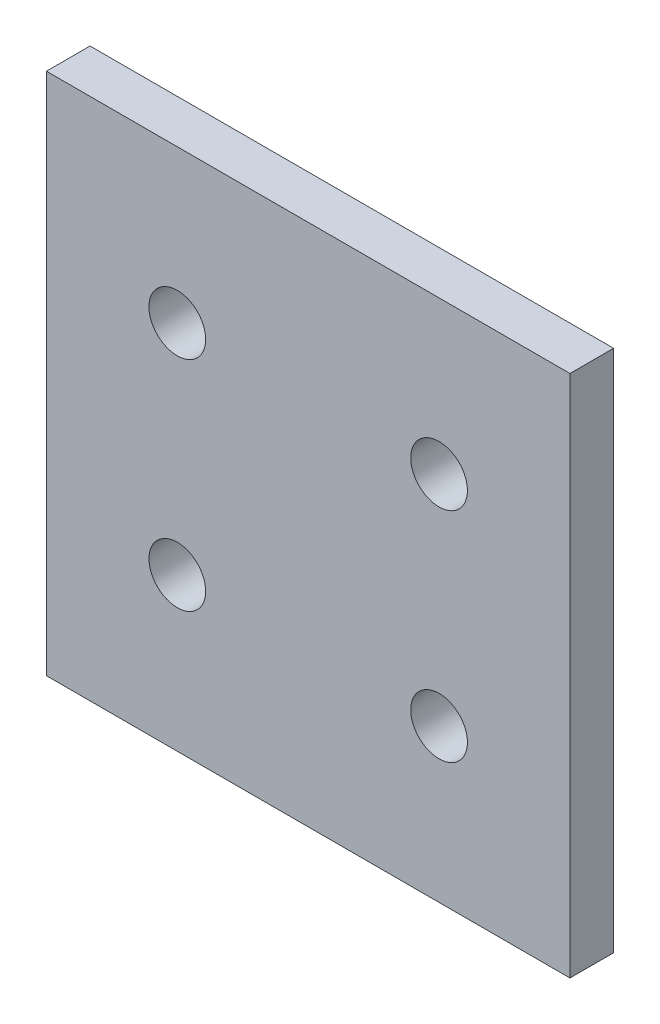
from build123d import *

# Parameters (mm, degrees)
SKETCH_1_W      = 120
SKETCH_1_H      = 120
SKETCH_1_R      = 6.5
EXTRUDE_1_DEPTH = 10


with BuildPart() as part:
    # 草图1 → 凸台-拉伸1 (new body)
    with BuildSketch(Plane.XY):
        with Locations((60, 60)):
            Rectangle(SKETCH_1_W, SKETCH_1_H)
        with Locations((90, 35)):
            Circle(SKETCH_1_R, mode=Mode.SUBTRACT)
        with Locations((30, 85)):
            Circle(SKETCH_1_R, mode=Mode.SUBTRACT)
        with Locations((90, 85)):
            Circle(SKETCH_1_R, mode=Mode.SUBTRACT)
        with Locations((30, 35)):
            Circle(SKETCH_1_R, mode=Mode.SUBTRACT)
    extrude(amount=EXTRUDE_1_DEPTH)


solid = part.part
